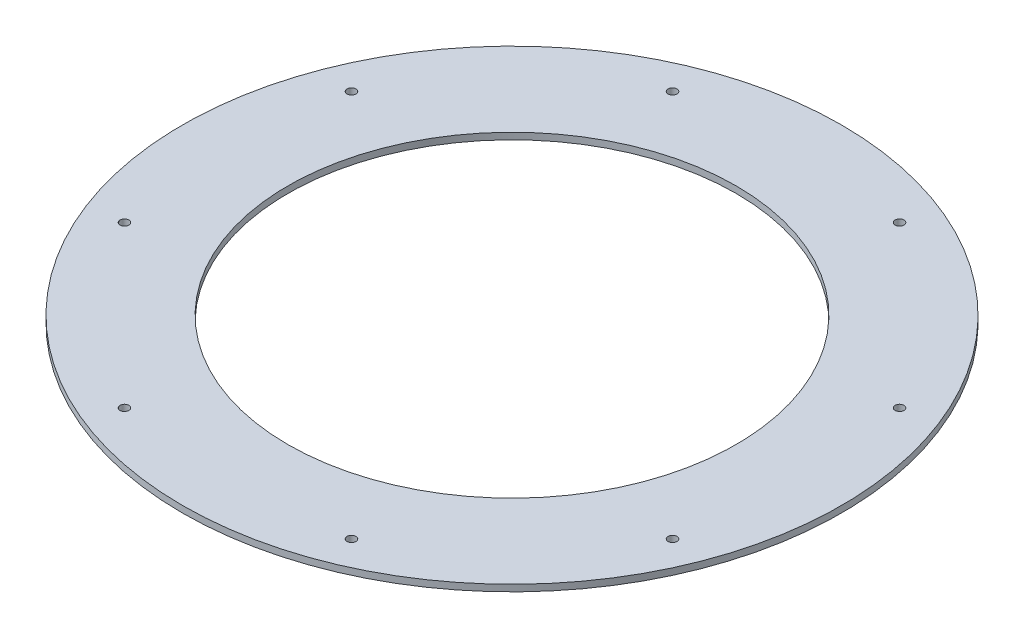
SolidWorks part; units mm, degrees
material "Q235B"
ref_plane "Front Plane" through (0, 0, 0) normal (0, 0, 1) x (1, 0, 0)
ref_plane "Top Plane" through (0, 0, 0) normal (0, 1, 0) x (1, 0, 0)
ref_plane "Right Plane" through (0, 0, 0) normal (1, 0, 0) x (0, 0, -1)
sketch "Sketch1" plane through (0, 0, 0) normal (0, 1, 0) x (1, 0, 0)
  circle A0 centre (0, 0) radius 500
  circle A1 centre (0, 0) radius 340
  dimension "D1" = 1000
  dimension "D2" = 680
extrude "Boss-Extrude1" add sketch "Sketch1" along normal mid plane 10
hole_wizard "Ø13.5 (13.5) Diameter Hole1" positions "Sketch2" profile "Sketch3" hole size "Ø13.5" standard "GB" end condition up to next
sketch "Sketch2" plane through (0, 5, 0) normal (0, 1, 0) x (1, 0, 0)
  line L0 (0, 0) -> (0, 450) construction
  circle A0 centre (0, 0) radius 450 construction
  point P0 (172.2075, 415.7458)
  point P73 (415.7458, 172.2075)
  point P74 (415.7458, -172.2075)
  point P75 (172.2075, -415.7458)
  point P76 (-172.2075, -415.7458)
  point P77 (-415.7458, -172.2075)
  point P78 (-415.7458, 172.2075)
  point P79 (-172.2075, 415.7458)
  dimension "D1" = 900
  dimension "D2" = 8
sketch "Sketch3" plane through (172.2075, 5, -415.7458) normal (1, 0, 0) x (0, 0, 1)
  line L0 (0, 0) -> (0, 10)
  line L1 (0, 10) -> (6.75, 10)
  line L2 (6.75, 10) -> (6.75, 0)
  line L5 (6.75, 0) -> (0, 0)
  line L11 (0, -6.35) -> (0, 107.95) construction
  dimension "通孔孔直径" = 13.5
  dimension "通孔孔深度" = 10
